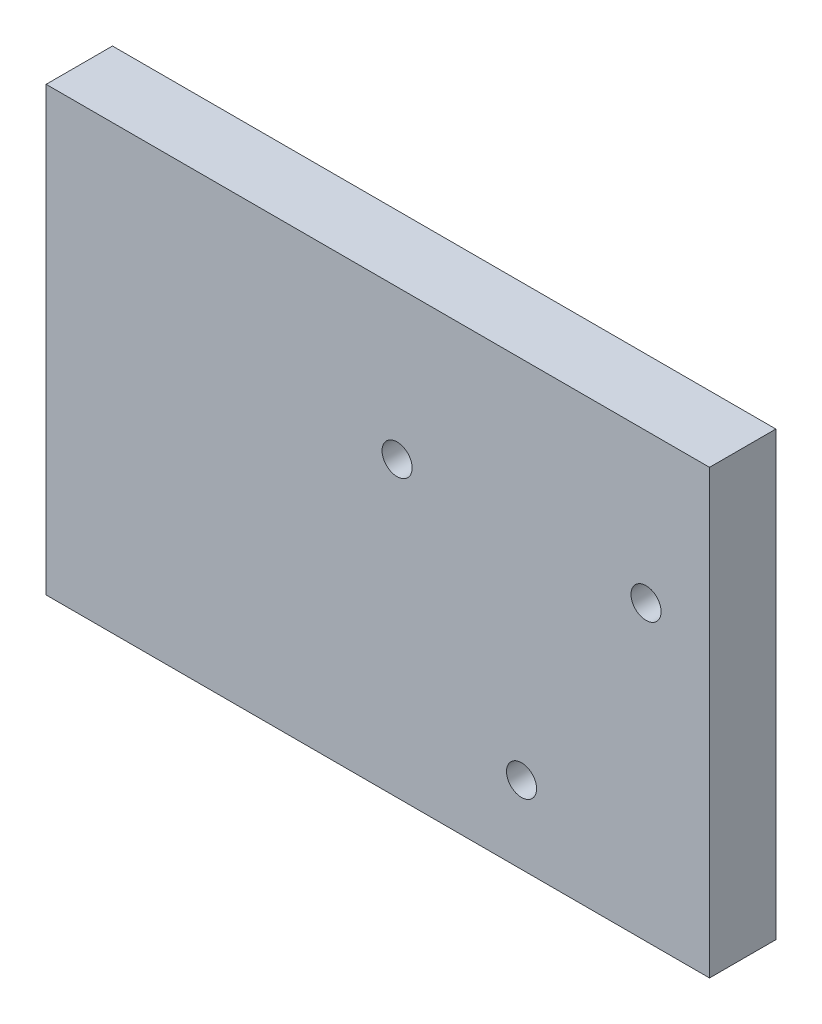
SolidWorks part; units mm, degrees
material "1023 碳钢板 (SS)"
ref_plane "Front Plane" through (0, 0, 0) normal (0, 0, 1) x (1, 0, 0)
ref_plane "Top Plane" through (0, 0, 0) normal (0, 1, 0) x (1, 0, 0)
ref_plane "Right Plane" through (0, 0, 0) normal (1, 0, 0) x (0, 0, -1)
sketch "Sketch1" plane through (0, 0, 0) normal (0, 0, 1) x (1, 0, 0)
  line L1 (-75, 50) -> (75, 50)
  line L2 (-75, 50) -> (-75, -50)
  line L3 (-75, -50) -> (75, -50)
  line L4 (75, 50) -> (75, -50)
  line L5 (-75, 50) -> (75, -50) construction
  line L6 (-75, -50) -> (75, 50) construction
  point P0 (0, 0)
  dimension "D1" = 150
  dimension "D2" = 100
extrude "Boss-Extrude1" add sketch "Sketch1" along normal blind 15
sketch "Sketch3" plane through (0, 0, 15) normal (0, 0, 1) x (1, 0, 0)
  line L0 (75, -50) -> (75, 50) construction
  line L1 (4.3542, 16.25) -> (32.5, 0) construction
  line L2 (32.5, 0) -> (60.6458, 16.25) construction
  line L3 (32.5, 0) -> (32.5, -32.5) construction
  circle A0 centre (32.5, 0) radius 32.5 construction
  circle A1 centre (32.5, -32.5) radius 4.8104
  circle A2 centre (4.3542, 16.25) radius 4.8862
  circle A3 centre (60.6458, 16.25) radius 3.8535
  dimension "D1" = 65
  dimension "D2" = 42.5
  dimension "D3" = 120
  dimension "D4" = 120
hole_wizard "M8 Tapped Hole1" positions "Sketch4" profile "Sketch5" tap size "M8" standard "GB"
sketch "Sketch4" plane through (0, 0, 15) normal (0, 0, 1) x (1, 0, 0)
  point P0 (4.3542, 16.25)
  point P3 (60.6458, 16.25)
  point P6 (32.5, -32.5)
sketch "Sketch5" plane through (4.3542, 16.25, 15) normal (1, 0, 0) x (0, -1, 0)
  line L0 (0, 0) -> (0, 21.7929)
  line L1 (0, 21.7929) -> (3.4, 19.75)
  line L2 (3.4, 19.75) -> (3.4, 0)
  line L5 (3.4, 0) -> (0, 0)
  line L10 (0, 21.7929) -> (-3.4, 19.75) construction
  line L11 (0, -6.35) -> (0, 107.95) construction
  dimension "螺纹孔钻头直径" = 6.8
  dimension "螺纹孔钻头深度" = 19.75
  dimension "导头角度" = 118
cosmetic thread "CosmeticThread Hole thread1"
cosmetic thread "CosmeticThread Hole thread2"
cosmetic thread "CosmeticThread Hole thread3"
